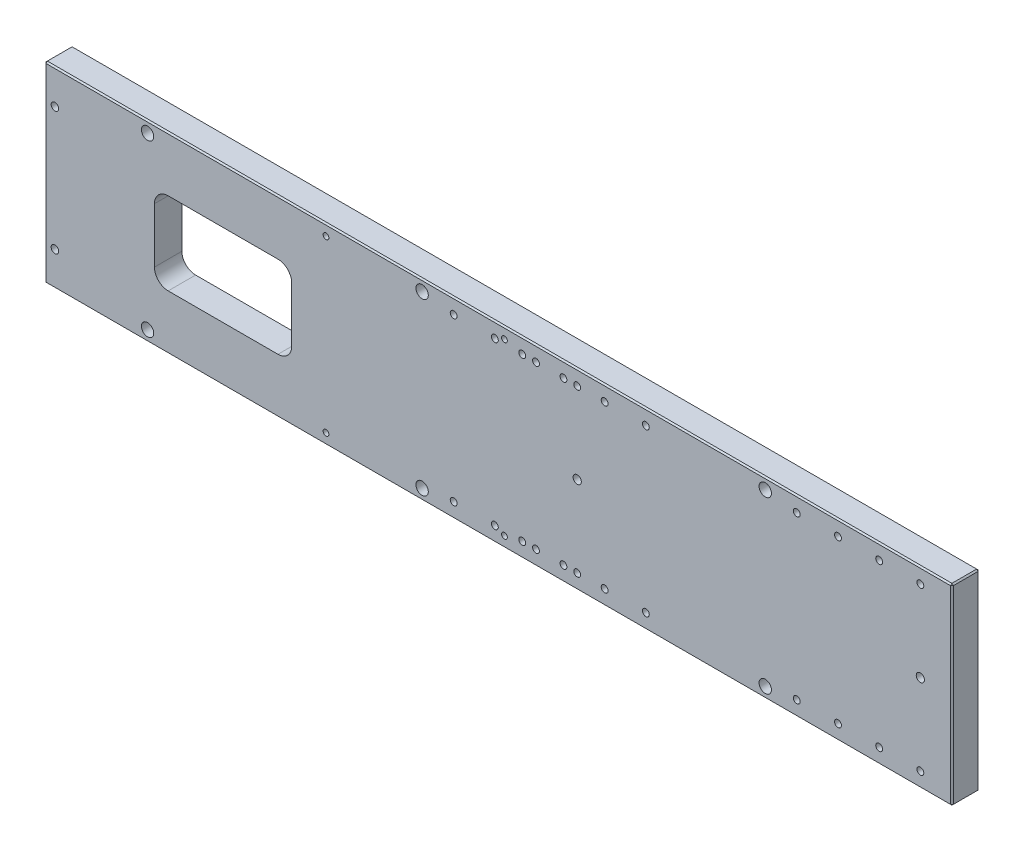
SolidWorks part; units mm, degrees
material "45#"
ref_plane "前视" through (0, 0, 0) normal (0, 0, 1) x (1, 0, 0)
ref_plane "上视" through (0, 0, 0) normal (0, 1, 0) x (1, 0, 0)
ref_plane "右视" through (0, 0, 0) normal (1, 0, 0) x (0, 0, -1)
sketch "草图1" plane through (0, 0, 0) normal (0, 0, 1) x (1, 0, 0)
  line L1 (-330.5, -70) -> (330.5, -70)
  line L2 (-330.5, -70) -> (-330.5, 70)
  line L3 (-330.5, 70) -> (330.5, 70)
  line L4 (330.5, -70) -> (330.5, 70)
  line L5 (-330.5, -70) -> (330.5, 70) construction
  line L6 (-330.5, 70) -> (330.5, -70) construction
  point P0 (0, 0)
  dimension "D1" = 661
  dimension "D2" = 140
extrude "凸台-拉伸1" add sketch "草图1" along normal blind 20
chamfer "倒角1" distance 1 angle 45 12 edges at (330.5, 70, 10) (-330.5, 70, 10) (-330.5, -70, 10) (0, 70, 0) (-330.5, 0, 0) (0, -70, 0) (330.5, 0, 0) (330.5, -70, 10) (0, -70, 20) (-330.5, 0, 20) (0, 70, 20) (330.5, 0, 20)
sketch "草图10" plane through (0, 0, 0) normal (0, 0, -1) x (-1, 0, 0)
  line L0 (-221, 0) -> (-32.8, 0) construction
  line L1 (-32.8, -17.5) -> (-32.8, 17.5) construction
  line L3 (-199.4, -37.5) -> (-54.4, -37.5)
  line L4 (-209.4, -27.5) -> (-209.4, 27.5)
  line L5 (-199.4, 37.5) -> (-54.4, 37.5)
  line L6 (-44.4, -27.5) -> (-44.4, 27.5)
  line L7 (-209.4, -37.5) -> (-44.4, 37.5) construction
  line L8 (-209.4, 37.5) -> (-44.4, -37.5) construction
  arc A0 (-54.4, 37.5) -> (-44.4, 27.5) centre (-54.4, 27.5) cw
  arc A1 (-54.4, -37.5) -> (-44.4, -27.5) centre (-54.4, -27.5) ccw
  arc A2 (-199.4, -37.5) -> (-209.4, -27.5) centre (-199.4, -27.5) cw
  arc A3 (-209.4, 27.5) -> (-199.4, 37.5) centre (-199.4, 27.5) cw
  point P5 (-126.9, 0)
  dimension "D3" = 10
  dimension "D1" = 165
  dimension "D2" = 75
extrude "切除-拉伸1" [suppressed] cut sketch "草图10" against normal through all
sketch "草图11" plane through (0, 0, 0) normal (0, 0, -1) x (-1, 0, 0)
  line L0 (330.5, 69) -> (330.5, -69) construction
  line L3 (-329.5, 70) -> (329.5, 70) construction
  line L4 (167.5, -30) -> (313.5, -30)
  line L5 (165.5, -28) -> (165.5, 43)
  line L6 (167.5, 45) -> (313.5, 45)
  line L7 (315.5, -28) -> (315.5, 43)
  line L8 (165.5, -30) -> (315.5, 45) construction
  line L9 (165.5, 45) -> (315.5, -30) construction
  arc A0 (313.5, 45) -> (315.5, 43) centre (313.5, 43) cw
  arc A1 (313.5, -30) -> (315.5, -28) centre (313.5, -28) ccw
  arc A2 (167.5, -30) -> (165.5, -28) centre (167.5, -28) cw
  arc A3 (165.5, 43) -> (167.5, 45) centre (167.5, 43) cw
  point P6 (240.5, 7.5)
  dimension "D3" = 2
  dimension "D1" = 75
  dimension "D2" = 150
  dimension "D4" = 15
  dimension "D5" = 25
extrude "切除-拉伸2" [suppressed] cut sketch "草图11" against normal through all
sketch "草图12" plane through (-330.5, 0, 0) normal (-1, 0, 0) x (0, 0, 1)
  line L0 (0, 0) -> (36.1441, 0) construction
  line L1 (10, 70) -> (10, -70) construction
  line L2 (1, 70) -> (19, 70) construction
  line L3 (19, -70) -> (1, -70) construction
  circle A0 centre (10, 25) radius 4.25
  circle A1 centre (10, -25) radius 4.25
  dimension "D1" = 8.5
  dimension "D2" = 25
extrude "切除-拉伸3" [suppressed] cut sketch "草图12" against normal up to surface (15 mm away)
hole_wizard "M5 螺纹孔1" positions "草图13" profile "草图14" tap size "M5" standard "GB" end condition through all
sketch "草图13" plane through (0, 0, 20) normal (0, 0, 1) x (1, 0, 0)
  line L0 (329.5, -70) -> (-329.5, -70) construction
  line L1 (-329.5, 70) -> (329.5, 70) construction
  line L2 (-330.5, -69) -> (-330.5, 69) construction
  point P0 (4.5, 62)
  point P2 (4.5, -62)
  point P4 (-125.5, 62)
  point P6 (-125.5, -62)
  point P8 (-255.5, -62)
  point P10 (-255.5, 62)
  dimension "D1" = 8
  dimension "D2" = 8
  dimension "D3" = 75
  dimension "D4" = 130
  dimension "D5" = 130
sketch "草图14" plane through (4.5, 62, 20) normal (1, 0, 0) x (0, -1, 0)
  line L0 (0, 0) -> (0, 20)
  line L1 (0, 20) -> (2.1, 20)
  line L2 (2.1, 20) -> (2.1, 0)
  line L5 (2.1, 0) -> (0, 0)
  line L11 (0, -6.35) -> (0, 107.95) construction
  dimension "通孔螺纹孔钻头直径" = 4.2
  dimension "通孔螺纹孔钻头深度" = 20
cosmetic thread "孔螺蚊线1" parameters "D2"=5
cosmetic thread "孔螺蚊线2" parameters "D2"=5
cosmetic thread "孔螺蚊线3" parameters "D2"=5
cosmetic thread "孔螺蚊线4" parameters "D2"=5
cosmetic thread "孔螺蚊线5" parameters "D2"=5
cosmetic thread "孔螺蚊线6" parameters "D2"=5
hole_wizard "M6 螺纹孔1" positions "草图16" profile "草图17" tap size "M6" standard "GB" end condition through all
sketch "草图16" plane through (0, 0, 20) normal (0, 0, 1) x (1, 0, 0)
  line L0 (330.5, 69) -> (330.5, -69) construction
  line L1 (57.5, 59) -> (395.5454, 59) construction
  point P2 (307.5, -59)
  point P4 (107.5, -59)
  point P6 (57.5, -59)
  point P8 (57.5, 59)
  point P10 (107.5, 59)
  point P12 (307.5, 59)
  point P24 (277.5, -59)
  point P25 (77.5, -59)
  point P26 (27.5, -59)
  point P27 (27.5, 59)
  point P28 (77.5, 59)
  point P29 (277.5, 59)
  point P30 (247.5, -59)
  point P31 (47.5, -59)
  point P32 (-2.5, -59)
  point P33 (-2.5, 59)
  point P34 (47.5, 59)
  point P35 (247.5, 59)
  point P36 (217.5, -59)
  point P37 (17.5, -59)
  point P38 (-32.5, -59)
  point P39 (-32.5, 59)
  point P40 (17.5, 59)
  point P41 (217.5, 59)
  dimension "D1" = 23
  dimension "D2" = 200
  dimension "D3" = 50
  dimension "D5" = 30
  dimension "D4" = 4
sketch "草图17" plane through (307.5, -59, 20) normal (1, 0, 0) x (0, -1, 0)
  line L0 (0, 0) -> (0, 20)
  line L1 (0, 20) -> (2.5, 20)
  line L2 (2.5, 20) -> (2.5, 0)
  line L5 (2.5, 0) -> (0, 0)
  line L11 (0, -6.35) -> (0, 107.95) construction
  dimension "通孔螺纹孔钻头直径" = 5
  dimension "通孔螺纹孔钻头深度" = 20
cosmetic thread "孔螺蚊线7" parameters "D2"=6
cosmetic thread "孔螺蚊线8" parameters "D2"=6
cosmetic thread "孔螺蚊线9" parameters "D2"=6
cosmetic thread "孔螺蚊线10" parameters "D2"=6
cosmetic thread "孔螺蚊线11" parameters "D2"=6
cosmetic thread "孔螺蚊线12" parameters "D2"=6
cosmetic thread "孔螺蚊线13" parameters "D2"=6
cosmetic thread "孔螺蚊线14" parameters "D2"=6
cosmetic thread "孔螺蚊线15" parameters "D2"=6
cosmetic thread "孔螺蚊线16" parameters "D2"=6
cosmetic thread "孔螺蚊线17" parameters "D2"=6
cosmetic thread "孔螺蚊线18" parameters "D2"=6
cosmetic thread "孔螺蚊线19" parameters "D2"=6
cosmetic thread "孔螺蚊线20" parameters "D2"=6
cosmetic thread "孔螺蚊线21" parameters "D2"=6
cosmetic thread "孔螺蚊线22" parameters "D2"=6
cosmetic thread "孔螺蚊线23" parameters "D2"=6
cosmetic thread "孔螺蚊线24" parameters "D2"=6
cosmetic thread "孔螺蚊线27" parameters "D2"=6
cosmetic thread "孔螺蚊线28" parameters "D2"=6
cosmetic thread "孔螺蚊线31" parameters "D2"=6
cosmetic thread "孔螺蚊线32" parameters "D2"=6
cosmetic thread "孔螺蚊线33" parameters "D2"=6
cosmetic thread "孔螺蚊线34" parameters "D2"=6
sketch "草图18" plane through (0, 0, 20) normal (0, 0, 1) x (1, 0, 0)
  line L0 (330.5, 69) -> (330.5, -69) construction
  circle A0 centre (307.5, 0) radius 3
  circle A1 centre (57.5, 0) radius 3
  dimension "D2" = 250
  dimension "D1" = 23
extrude "切除-拉伸4" cut sketch "草图18" against normal through all
hole_wizard "打孔尺寸(%根据)内六角圆柱头螺钉的类型1" positions "草图19" profile "草图20" counterbore size "M5" standard "GB" end condition through all
sketch "草图19" plane through (0, 0, 0) normal (0, 0, -1) x (-1, 0, 0)
  point P3 (323, 45)
  point P5 (323, -45)
sketch "草图20" plane through (-323, 45, 0) normal (1, 0, 0) x (0, 1, 0)
  line L0 (0, 0) -> (0, 20)
  line L1 (0, 20) -> (2.75, 20)
  line L3 (2.75, 20) -> (2.75, 5.7)
  line L4 (5, 5.7) -> (2.75, 5.7)
  line L5 (5, 5.7) -> (5, 0.525)
  line L6 (5, 0.525) -> (5.525, 0)
  line L7 (5.525, 0) -> (0, 0)
  line L8 (-5, 0.525) -> (-5.525, 0) construction
  line L11 (0, -6.35) -> (0, 107.95) construction
  dimension "通孔孔直径" = 5.5
  dimension "通孔孔深度" = 20
  dimension "柱形沉头孔直径" = 10
  dimension "柱形沉头孔深度" = 5.7
  dimension "近端锥形沉头孔直径" = 11.05
  dimension "近端锥形沉头孔角度" = 90
hole_wizard "Hole1" positions "Point_Sketch" profile "Profil_Sketch" counterbore size "M6" standard "ISO" end condition through all
sketch "Point_Sketch" plane through (-242.6309, -61.065, 0) normal (0, 0, 1) x (-1, 0, 0)
  line L0 (86.8691, -61.065) -> (-142.3532, -61.065) construction
  line L1 (86.8691, 7.935) -> (86.8691, -130.065) construction
  point P0 (12.8691, 0.935)
  point P2 (-187.1309, 0.935)
  point P4 (-437.1309, 0.935)
  point P18 (-437.1309, -123.065)
  point P19 (-187.1309, -123.065)
  point P20 (12.8691, -123.065)
sketch "Profil_Sketch" plane through (-255.5, -62, 0) normal (1, 0, 0) x (0, 1, 0)
  line L0 (0, 0) -> (0, 20)
  line L1 (0, 20) -> (4.5, 20)
  line L3 (4.5, 20) -> (4.5, 8.5)
  line L4 (4.5, 8.5) -> (7.5, 8.5)
  line L5 (7.5, 8.5) -> (7.5, 0)
  line L7 (7.5, 0) -> (0, 0)
  line L11 (0, -6.35) -> (0, 107.95) construction
  dimension "Diameter" = 9
  dimension "Thru Hole Depth" = 20
  dimension "L1" = 8.5
other "usin_LS160_M8x25-SH<1>"
sketch "草图21" plane through (0, 0, 0) normal (0, 0, -1) x (-1, 0, 0)
  line L0 (0, 0) -> (391.3331, 0) construction
  line L1 (150.5, 30) -> (250.5, 30)
  line L2 (150.5, 30) -> (150.5, -30)
  line L3 (150.5, -30) -> (250.5, -30)
  line L4 (250.5, 30) -> (250.5, -30)
  line L5 (330.5, 69) -> (330.5, -69) construction
  dimension "D1" = 80
  dimension "D2" = 60
  dimension "D3" = 100
extrude "切除-拉伸5" cut sketch "草图21" against normal through all
fillet "圆角2" radius 10 4 edges at (-250.5, 30, 10) (-250.5, -30, 10) (-150.5, 30, 10) (-150.5, -30, 10)
